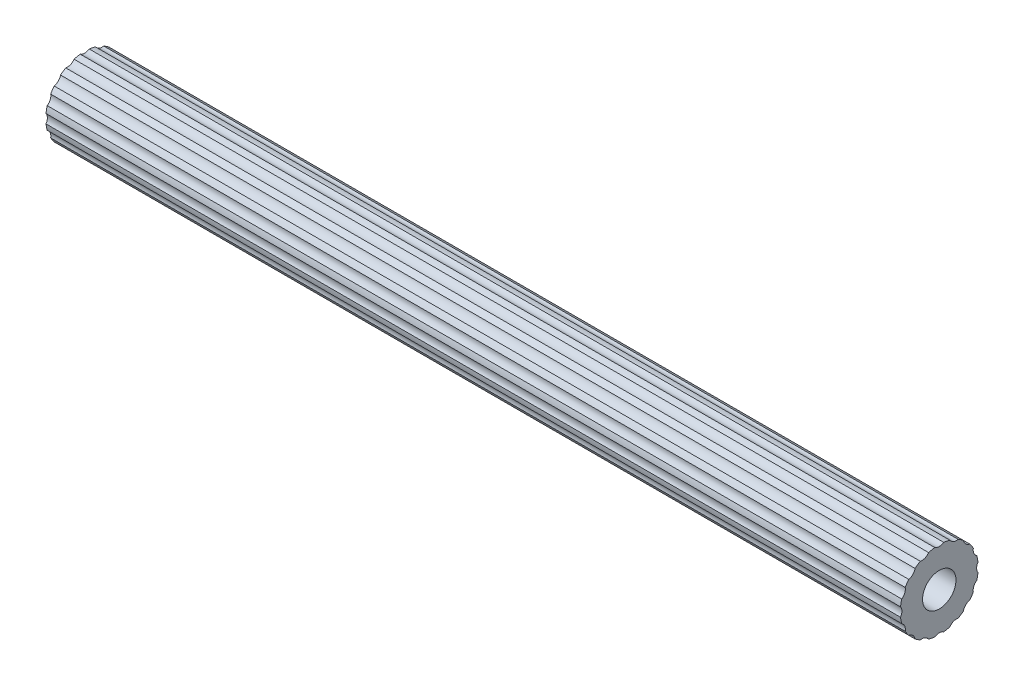
from build123d import *

# Parameters (mm, degrees)
SKETCH1_R                = 35
SKETCH1_R_2              = 15
BOSS_EXTRUDE2_DEPTH      = 767
SKETCH2_R                = 7.203487768
CUT_EXTRUDE1_DEPTH       = 767
PATTERN_CIRCULAR_1_COUNT = 16


with BuildPart() as part:
    # Sketch1 → Boss-Extrude2 (new body)
    with BuildSketch(Plane(origin=(0, 0, 0), x_dir=(0, 0, -1), z_dir=(1, 0, 0))):
        Circle(SKETCH1_R)
        Circle(SKETCH1_R_2, mode=Mode.SUBTRACT)
    extrude(amount=BOSS_EXTRUDE2_DEPTH)

    # Sketch2 → Cut-Extrude1 (cut)
    with BuildSketch(Plane.ZY):
        with Locations((0, 40.740922714)):
            Circle(SKETCH2_R)
    cut_extrude1 = extrude(amount=-CUT_EXTRUDE1_DEPTH, mode=Mode.SUBTRACT)

    # Pattern(Circular)1: Cut-Extrude1 ×16 about axis
    pattern_circular_1_axis = Axis((0, 0, 0), (1, 0, 0))
    for i in range(1, PATTERN_CIRCULAR_1_COUNT):
        add(cut_extrude1.rotate(pattern_circular_1_axis, i * 360 / PATTERN_CIRCULAR_1_COUNT), mode=Mode.SUBTRACT)


solid = part.part
